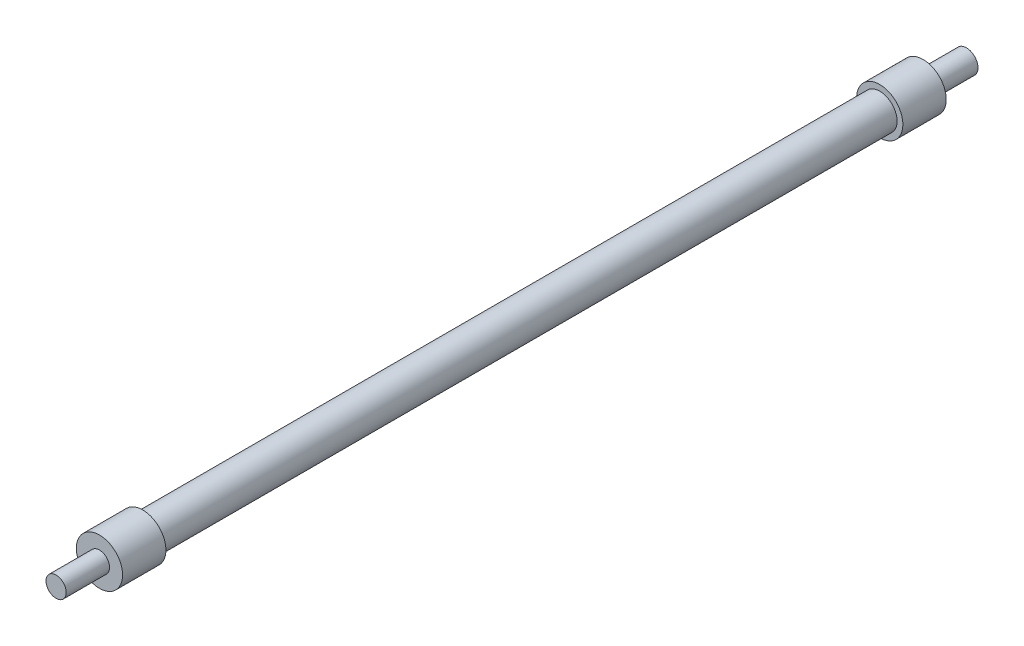
SolidWorks part; units mm, degrees
ref_plane "前视基准面" through (0, 0, 0) normal (0, 0, 1) x (1, 0, 0)
ref_plane "上视基准面" through (0, 0, 0) normal (0, 1, 0) x (1, 0, 0)
ref_plane "右视基准面" through (0, 0, 0) normal (1, 0, 0) x (0, 0, -1)
sketch "草图1" plane through (0, 0, 0) normal (0, 0, 1) x (1, 0, 0)
  circle A0 centre (0, 0) radius 4
  dimension "D1" = 8
extrude "凸台-拉伸1" add sketch "草图1" along normal blind 15
cosmetic thread "装饰螺纹线1" parameters "D1"=15, "D2"=6
sketch "草图2" plane through (0, 0, 15) normal (0, 0, 1) x (1, 0, 0)
  circle A0 centre (0, 0) radius 6
  dimension "D1" = 12
extrude "凸台-拉伸2" add sketch "草图2" along normal blind 270
sketch "草图3" plane through (0, 0, 15) normal (0, 0, -1) x (-1, 0, 0)
  circle A0 centre (0, 0) radius 8
  dimension "D1" = 16
extrude "凸台-拉伸3" add sketch "草图3" against normal blind 15
sketch "草图4" plane through (0, 0, 285) normal (0, 0, 1) x (1, 0, 0)
  circle A0 centre (0, 0) radius 8 construction
  circle A1 centre (0, 0) radius 8
extrude "凸台-拉伸4" add sketch "草图4" along normal blind 15
sketch "草图5" plane through (0, 0, 300) normal (0, 0, 1) x (1, 0, 0)
  circle A0 centre (0, 0) radius 3.5
  dimension "D1" = 7
extrude "凸台-拉伸5" add sketch "草图5" along normal blind 15
cosmetic thread "装饰螺纹线2" parameters "D1"=15, "D2"=6
